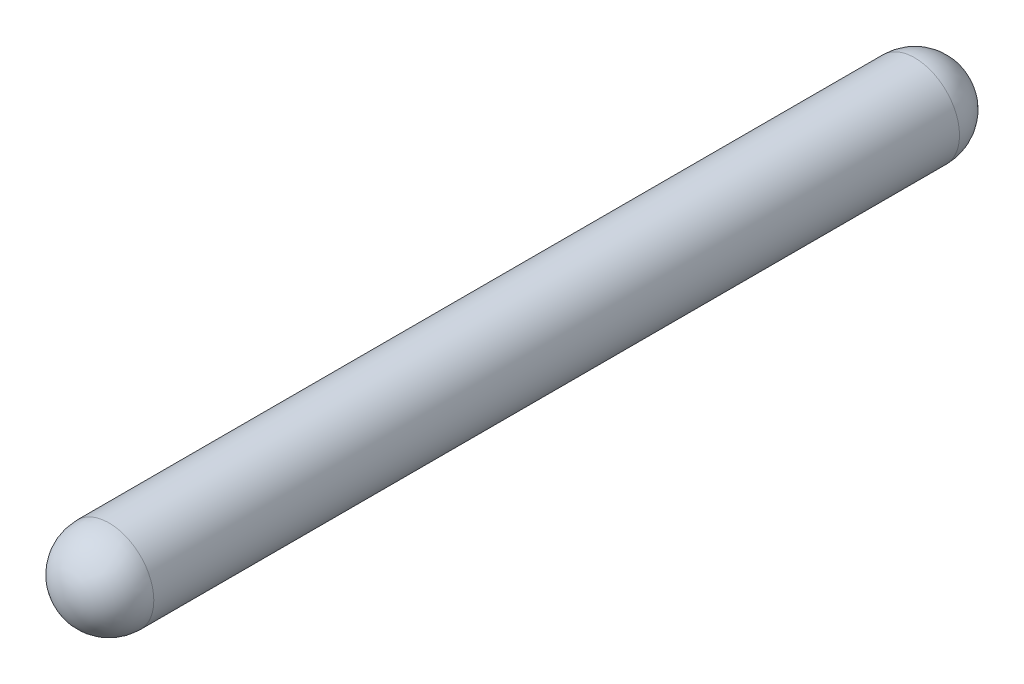
from build123d import *

# Parameters (mm, degrees)
BOSS_EXTRUDE1_START = -15
SKETCH1_R           = 1
BOSS_EXTRUDE1_DEPTH = 10
FILLET1_R           = 1


with BuildPart() as part:
    # Sketch1 → Boss-Extrude1 (new, symmetric)
    with BuildSketch(Plane.XY.offset(BOSS_EXTRUDE1_START)):
        with Locations((-91.3, 42)):
            Circle(SKETCH1_R)
    extrude(amount=BOSS_EXTRUDE1_DEPTH, both=True)

    # Fillet1
    fillet1_edges = [part.edges().sort_by_distance(p)[0] for p in [
        (-92.3, 42, -5),
        (-92.3, 42, -25),
    ]]
    fillet(fillet1_edges, radius=FILLET1_R)


solid = part.part
